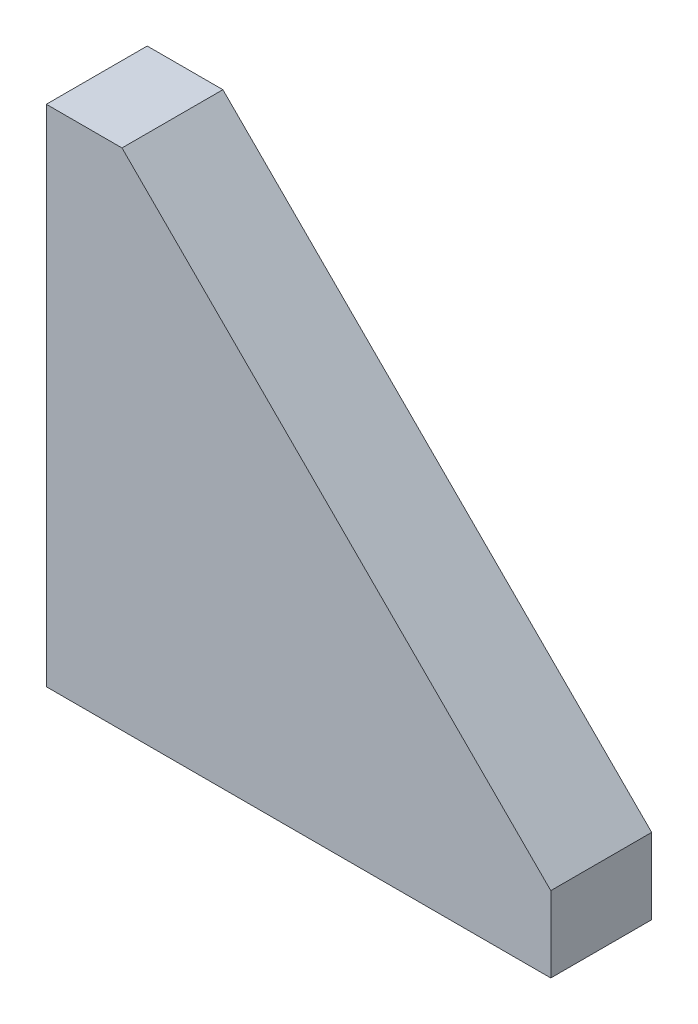
from build123d import *

# Parameters (mm, degrees)
BOSS_EXTRUDE1_DEPTH = 20


with BuildPart() as part:
    # Sketch1 → Boss-Extrude1 (new body)
    with BuildSketch(Plane.XY):
        Polygon((0, 0), (0, 100), (15, 100), (100, 15), (100, 0), align=None)
    extrude(amount=BOSS_EXTRUDE1_DEPTH)


solid = part.part
